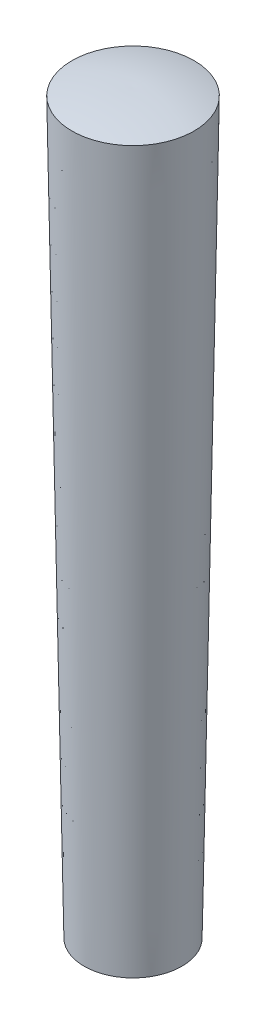
SolidWorks part; units mm, degrees
ref_plane "Front" through (0, 0, 0) normal (0, 0, 1) x (1, 0, 0)
ref_plane "Top" through (0, 0, 0) normal (0, 1, 0) x (1, 0, 0)
ref_plane "Right" through (0, 0, 0) normal (1, 0, 0) x (0, 0, -1)
sketch "Sketch1" plane through (0, 0, 0) normal (0, 0, 1) x (1, 0, 0)
  line L1 (-3.6161, 37.0258) -> (-2.896, -6.1751)
  line L2 (0, 0) -> (0, 30.0622)
  line L3 (0, 30.0622) -> (0, 37.4766)
  line L6 (0, 0) -> (0, -6.6693)
  arc A0 (0, 37.4766) -> (-3.6161, 37.0258) centre (-0.2738, 24.9441) ccw
  arc A1 (0, -6.6693) -> (-2.896, -6.1751) centre (0.1951, 3.2065) cw
revolve "Revolve1" add sketch "Sketch1" angle 360 about L2
scale "Scale 1" bodies to scale 101 scale about centroid uniform scaling yes scale factor 1.875
